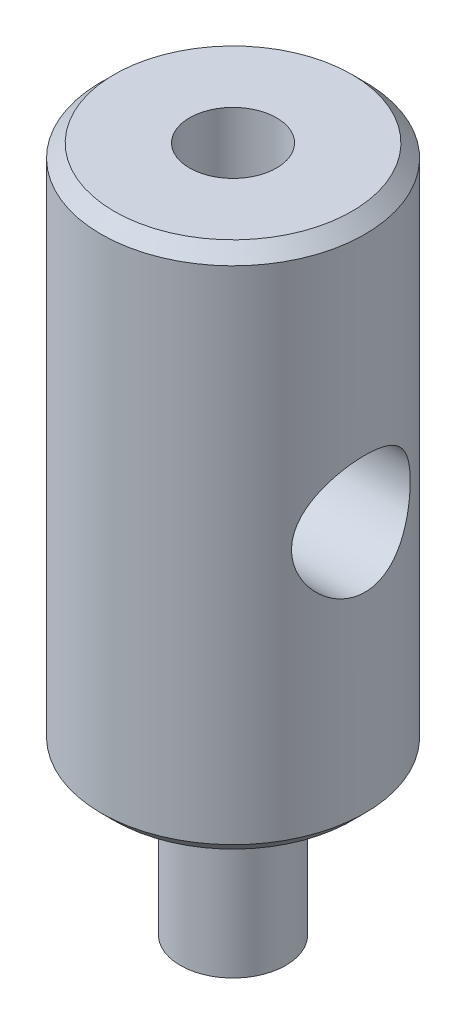
from build123d import *

# Parameters (mm, degrees)
SKETCH_1_R               = 5
EXTRUDE_1_DEPTH          = 10
SKETCH_2_R               = 2
EXTRUDE_2_DEPTH          = 6
SKETCH_3_W               = 0.3
SKETCH_3_H               = 0.5
HOLE_WIZARD_M4_1_D       = 3.3
HOLE_WIZARD_M4_1_DEPTH   = 10.1
HOLE_WIZARD_M4_1_TIP     = 0.991420021
CHAMFER_1_SIZE           = 0.5
CUT_EXTRUDE_1_DEPTH      = 18.492855685
CUT_EXTRUDE_1_DEPTH_BACK = 18.492855685
SKETCH_6_R               = 2.25


with BuildPart() as part:
    # 草图1 → 凸台-拉伸1 (new, symmetric)
    with BuildSketch(Plane(origin=(0, 0, 0), x_dir=(1, 0, 0), z_dir=(0, 1, 0))):
        with Locations(Location((0, 0, 0), (0, 0, 270))):
            Circle(SKETCH_1_R)
    extrude(amount=EXTRUDE_1_DEPTH, both=True)

    # 草图2 → 凸台-拉伸2 (add)
    with BuildSketch(Plane.XZ.offset(10)):
        with Locations(Location((0, 0, 0), (0, 0, 90))):
            Circle(SKETCH_2_R)
    extrude(amount=EXTRUDE_2_DEPTH)

    # 草图3 → 切除-旋转1 (revolve, cut)
    with BuildSketch(Plane.XY, mode=Mode.PRIVATE) as cut_revolve_1_sk:
        with Locations((1.85, -10.25)):
            Rectangle(SKETCH_3_W, SKETCH_3_H)
    revolve(cut_revolve_1_sk.sketch.rotate(Axis((0, 0, 0), (0, -1, 0)), 90), axis=Axis((0, 0, 0), (0, -1, 0)), mode=Mode.SUBTRACT)

    # M4 螺纹孔1
    with Locations(Plane(origin=(0, 10, 0), x_dir=(1, 0, 0), z_dir=(0, 1, 0))):
        with Locations((0, 0)):
            Hole(HOLE_WIZARD_M4_1_D / 2, depth=HOLE_WIZARD_M4_1_DEPTH)
            with Locations((0, 0, -(HOLE_WIZARD_M4_1_DEPTH + HOLE_WIZARD_M4_1_TIP / 2))):  # 118° drill point
                Cone(0, HOLE_WIZARD_M4_1_D / 2, HOLE_WIZARD_M4_1_TIP, mode=Mode.SUBTRACT)

    # 倒角1
    chamfer_1_edges = [part.edges().sort_by_distance(p)[0] for p in [
        (0, -10, -5),
        (0, 10, -5),
    ]]
    chamfer(chamfer_1_edges, length=CHAMFER_1_SIZE)

    # 草图6 → 切除-拉伸1 (cut, two sides: drawn at the far end of the back side and taken through both)
    with BuildSketch(Plane(origin=(0, 0, 0), x_dir=(0, 0, -1), z_dir=(1, 0, 0)).offset(-CUT_EXTRUDE_1_DEPTH_BACK)):
        Circle(SKETCH_6_R)
    extrude(amount=CUT_EXTRUDE_1_DEPTH + CUT_EXTRUDE_1_DEPTH_BACK, mode=Mode.SUBTRACT)


solid = part.part
